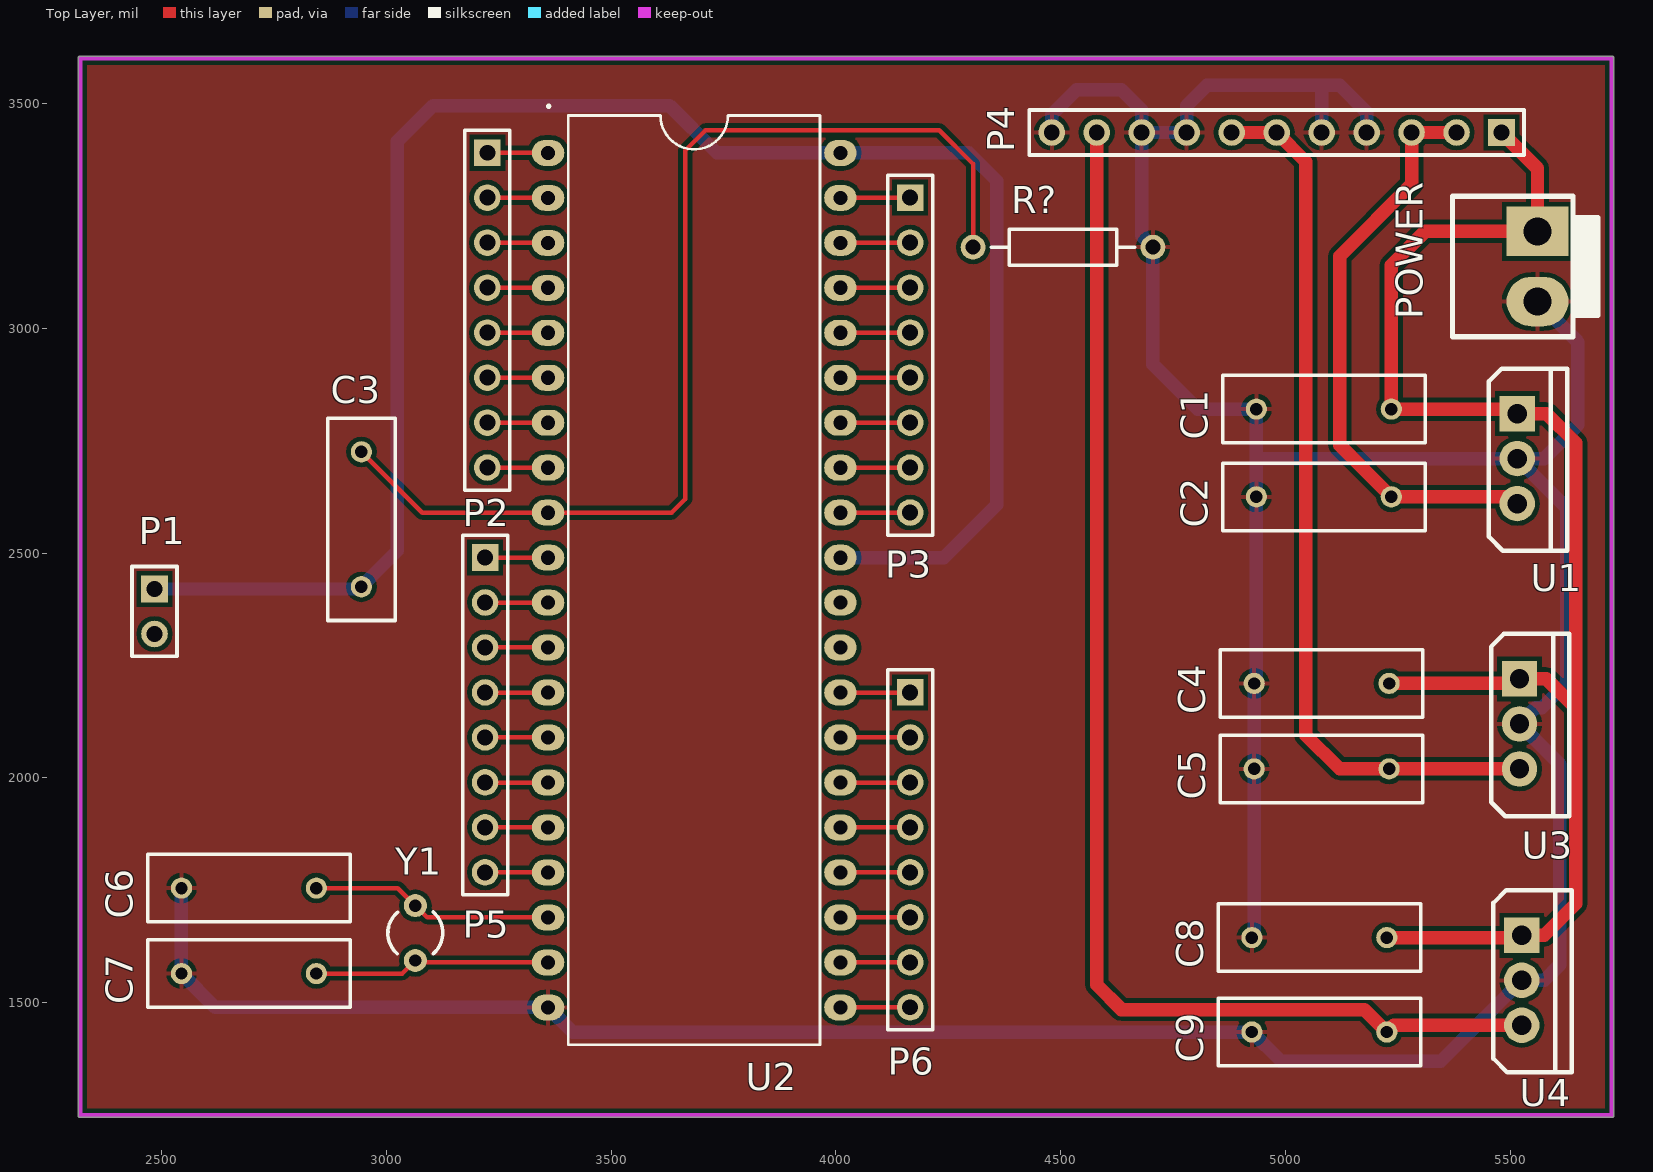
[diagram p0: Top Layer view]
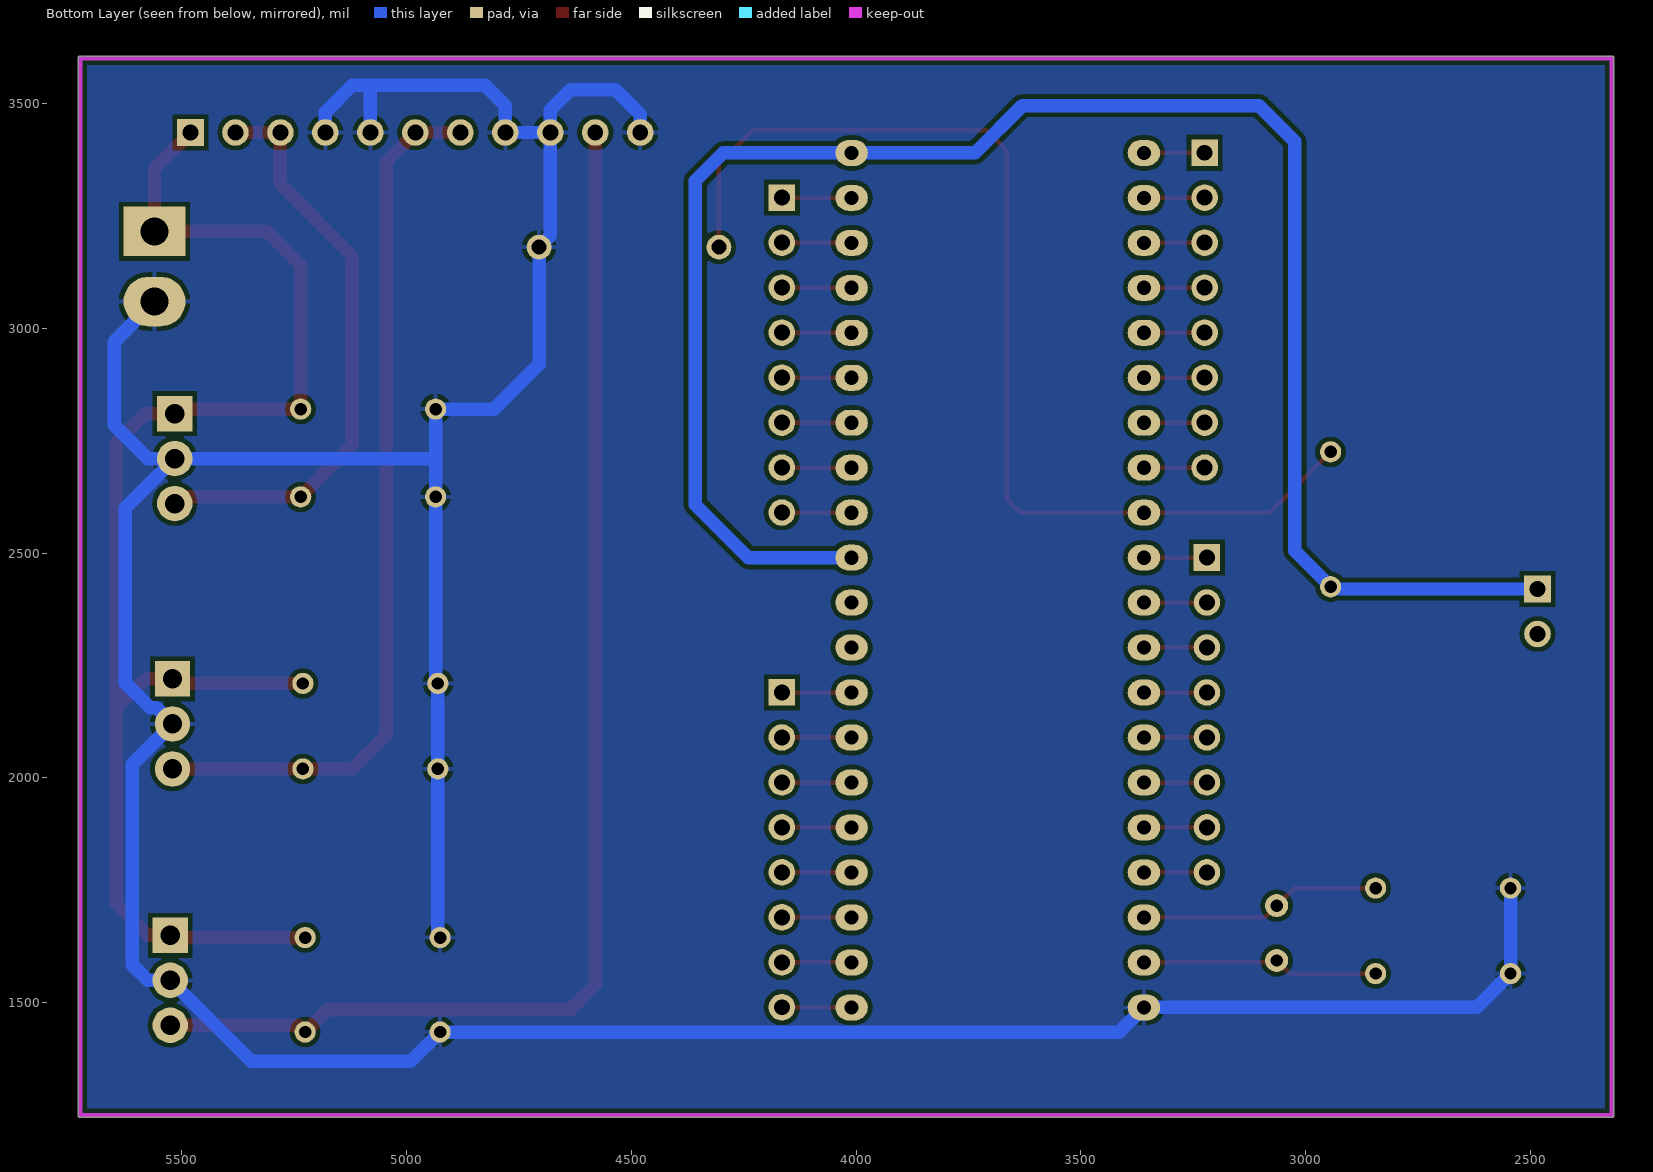
[diagram p1: Bottom Layer view, seen from below]
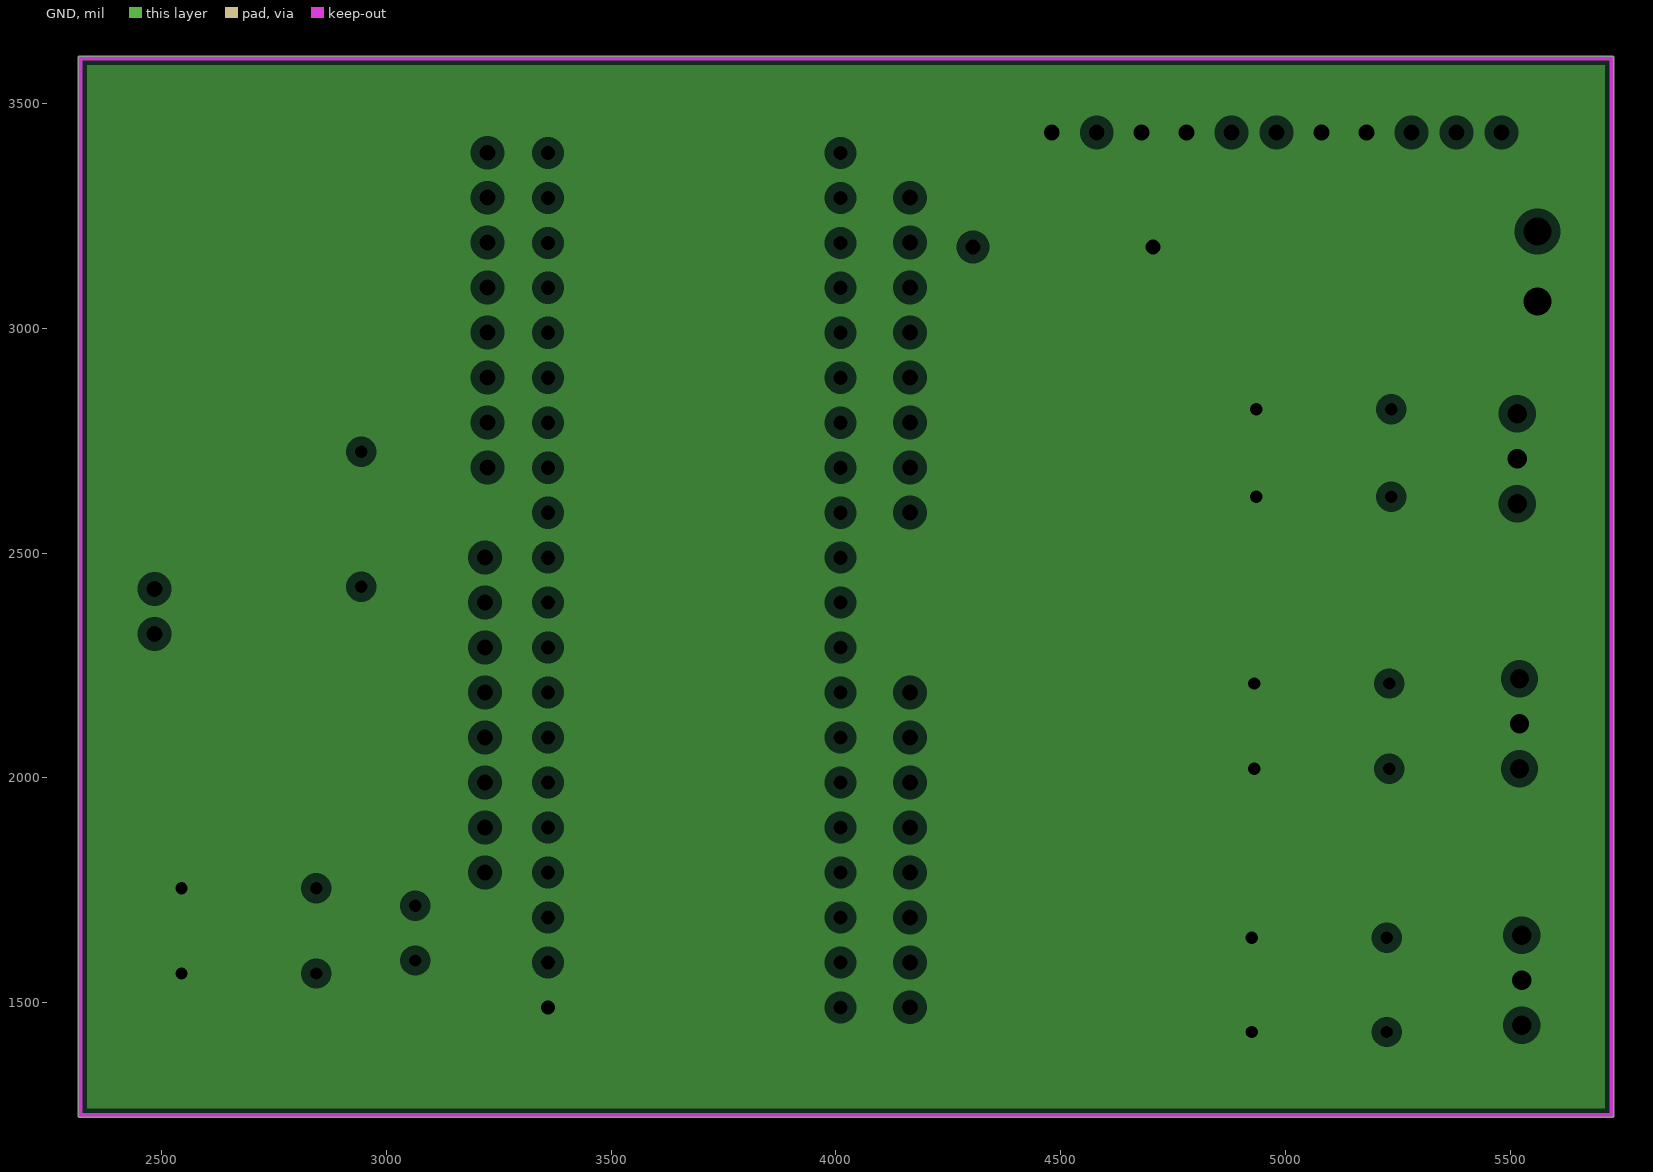
[diagram p2: GND, clearances drawn from the general rule]
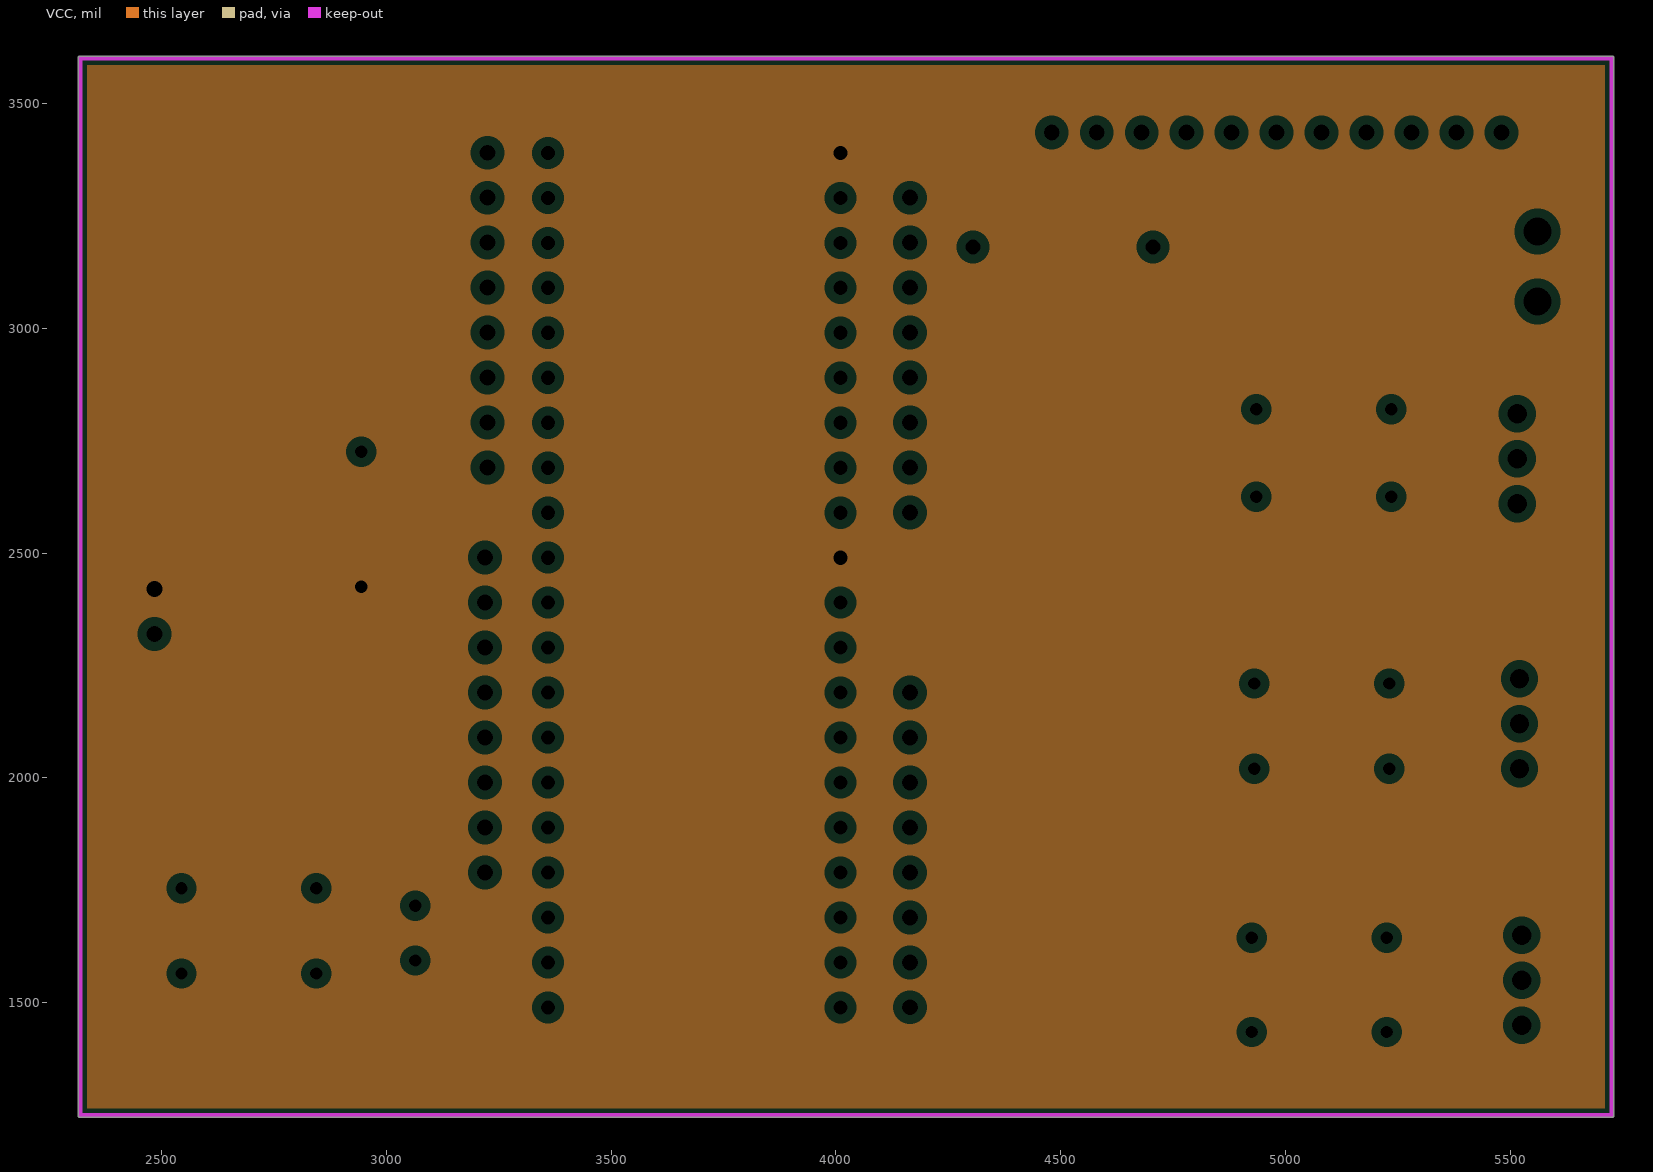
[diagram p3: VCC, clearances drawn from the general rule]
# Altium PCB MISC80518.PcbDoc
Units mil, origin at the board's own origin, x right, y up, seen from the top; angles counter-clockwise.
Board outline 3415.03 x 2360.03 mil, 4 copper layers (Top Layer, GND, VCC, Bottom Layer), stack 30.634 mil thick; 22 components, 41 nets, 118 pads, 0 vias.

## Layer stack, top to bottom
Top Solder: solder mask 0.4, Solder Resist, Dk 3.5
Top Layer: signal copper 1.4
Dielectric 1: core 10, FR-4, Dk 4.2
GND: plane copper 1.417, net GND
Dielectric 3: prepreg 5, Dk 4.2
VCC: plane copper 1.417, net VCC
Dielectric 2: core 10, Dk 4.2
Bottom Layer: signal copper 1.4
Bottom Solder: solder mask 0.4, Solder Resist, Dk 3.5

## Board outline
2314.99,1250 ccw(c2320,1250) 2320,1244.98 5725,1244.98 ccw(c5725,1250) 5730.02,1250 5730.02,3600 ccw(c5725,3600) 5725,3605.01 2320,3605.01 ccw(c2320,3600) 2314.99,3600

## Design rules (kind name [scope] priority, off if disabled: settings)
Clearance [All] p1: gap=10
MinimumSolderMaskSliver [All] p1: minsoldermaskwidth=0
PlaneClearance [All] p1: clearance=20
PlaneConnect [All] p1: planeconnectstyle=Relief reliefexpansion=20 reliefentries=4 reliefconductorwidth=10 reliefairgap=10
PolygonConnect [All] p1: connectstyle=Relief reliefconductorwidth=10 reliefentries=4 polygonreliefangle="90 Angle" airgapwidth=10
RoutingVias [All] p1: holewidth=28 width=50 viastyle="Through Hole" minholewidth=28 minwidth=50 maxholewidth=28 maxwidth=50
SilkToSilkClearance [All] p1: silktosilkclearance=0
SilkToSolderMaskClearance [IsPad] p1: minsilkscreentomaskgap=0 clearancetoexposedcopper=TRUE
SolderMaskExpansion [All] p1: expansion=4
Width [All] p1: maxlimit=50 minlimit=10 preferedwidth=10
25 further rules are at their usual default settings.

## Components (designator, comment, footprint, x,y, rotation, side; value= is the part's Value field where it differs from the comment)
C1 "0.33UF" RAD-0.3 5085,2820 r180 top
C2 "0.1UF" RAD-0.3 5085,2625 r180 top
C3 "10UF" RAD-0.3 2945,2575 r90 top
C4 "0.33UF" RAD-0.3 5080,2210 r180 top
C5 "0.1UF" RAD-0.3 5080,2020 r180 top
C6 "22pF" RAD-0.3 2695,1755 r180 top
C7 "22pF" RAD-0.3 2695,1565 r180 top
C8 "0.33UF" RAD-0.3 5075,1645 r180 top
C9 "0.1UF" RAD-0.3 5075,1435 r180 top
P1 "Header 2" HDR1X2 2485,2420 r270 top
P2 "Header 8" HDR1X8 3225,3390 r270 top
P3 "Header 8" HDR1X8 4165,3290 r270 top
P4 "Header 11" HDR1X11 5480,3435 r180 top
P5 "Header 8" HDR1X8 3220,2490 r270 top
P6 "Header 8" HDR1X8 4165,2190 r270 top
POWER "Terminal block" VH3.96-2A 5560,3215 r270 top
R? "10K" AXIAL-0.4 4505,3180 r180 top
U1 "LM7805" TO220A 5515,2710 r270 top
U2 "STC89C52RC" STC89C52RC 3685,2450 r270 top
U3 "LM7805" TO220A 5520,2120 r270 top
U4 "LM7806" TO220A 5525,1550 r270 top
Y1 "XTAL" R38 3065,1655 r180 top

## Footprints (in the part's own frame and the unit in brackets; to place one, negate y for a bottom-side part, rotate by r counter-clockwise, add the part's x,y. Pads: shape width x height; smd on the part's side, far side on the other; paste and mask are expansions set on the pad)
AXIAL-0.4 [mm] "Axial Device, Thru-Hole; 2 Leads; 0.4 in Pin Spacing"
  round 1.4 hole 0.85: 1(-5.08,0) 2(5.08,0)
  silkscreen extent -4.06,-1.02 4.06,1.02
HDR1X2 [mm] "Connector; Header; 2 Position"
  rect 1.5x1.5 hole 0.9: 1(0,0)
  round 1.5 hole 0.9: 2(2.54,0)
  silkscreen extent -1.27,-1.27 3.81,1.27
HDR1X8 [mm] "Connector; Header; 8 Position"
  rect 1.5x1.5 hole 0.9: 1(0,0)
  round 1.5 hole 0.9: 2(2.54,0) 3(5.08,0) 4(7.62,0) 5(10.16,0) 6(12.7,0) 7(15.24,0) 8(17.78,0)
  silkscreen extent -1.27,-1.27 19.05,1.27
HDR1X11 [mm] "Connector; Header; 11 Position"
  rect 1.5x1.5 hole 0.9: 1(0,0)
  round 1.5 hole 0.9: 2(2.54,0) 3(5.08,0) 4(7.62,0) 5(10.16,0) 6(12.7,0) 7(15.24,0) 8(17.78,0) 9(20.32,0) 10(22.86,0) 11(25.4,0)
  silkscreen extent -1.27,-1.27 26.67,1.27
R38 [mm] "Crystal, Thru-Hole; 2 Leads; Body 3.1 x 8.2 mm (Dia.xH)"
  round 1.3 hole 0.7: 1(0,1.55) 2(0,-1.55)
  silkscreen extent -1.55,-1.19 1.55,1.17
RAD-0.3 [mm] "Radial Cap, Thru-Hole; 2 Leads; 0.3 in Pin Spacing"
  round 1.2 hole 0.7: 1(-3.81,0) 2(3.81,0)
  silkscreen extent -5.71,-1.91 5.71,1.91
STC89C52RC [mm]
  oval 1.467x1.833 hole 0.8 paste+0 mask+0.051: 1(-23.868,-8.255) 2(-21.328,-8.255) 3(-18.788,-8.255) 4(-16.248,-8.255) 5(-13.708,-8.255) 6(-11.168,-8.255) 7(-8.628,-8.255) 8(-6.088,-8.255) 9(-3.548,-8.255) 10(-1.008,-8.255) 11(1.532,-8.255) 12(4.072,-8.255) 13(6.612,-8.255) 14(9.152,-8.255) 15(11.692,-8.255) 16(14.232,-8.255) 17(16.772,-8.255) 18(19.312,-8.255) 19(21.852,-8.255) 20(24.392,-8.255) 21(24.392,8.255) 22(21.852,8.255) 23(19.312,8.255) 24(16.772,8.255) 25(14.232,8.255) 26(11.692,8.255) 27(9.152,8.255) 28(6.612,8.255) 29(4.072,8.255) 30(1.532,8.255) 31(-1.008,8.255) 32(-3.548,8.255) 33(-6.088,8.255) 34(-8.628,8.255) 35(-11.168,8.255) 36(-13.708,8.255) 37(-16.248,8.255) 38(-18.788,8.255) 39(-21.328,8.255) 40(-23.868,8.255)
  silkscreen extent -26.58,-8.3 26.5,7.11
TO220A [mm] "220，3脚晶体管"
  rect 2x2 hole 1.1: 1(-2.54,0)
  round 2 hole 1.1: 2(0,0) 3(2.54,0)
  silkscreen extent -5.08,-1.6 5.21,2.82, body extent -5.08,-1.45 5.22,2.98, height 18.5
VH3.96-2A [mm]
  rect 2.8x3.5 hole 1.6: 1(0,0)
  oval 2.8x3.5 hole 1.6: 2(3.96,0)
  silkscreen extent -1.98,-4.8 5.94,3.4, body extent -1.98,-4.8 5.94,3.6, height 14.6

## Part data
C1 C2 C3 C4 C5 C6 C7 C8 C9: library part Cap, "Capacitor"
P1: "Header, 2-Pin"
P2 P3 P5 P6: "Header, 8-Pin"
P4: "Header, 11-Pin"
POWER: library part VH2
R?: library part Res2, "Resistor"
U4: library part LM7805
Y1: "Crystal Oscillator"

## Nets (pads, with @x,y where several pads share a name; then routed paths per layer and width w, separated by ;. In a path a pad name is that pad's centre, name@x,y a point inside that pad or via, vN(x,y) a via of type N, cw(c..) or ccw(c..) an arc to the next point about the centre after c; other vN are vias at no path point)
5V1: C2.1 P4.2 P4.3 U1.3 | length 1310.1
  Top Layer w30: P4.2 P4.3 5280,3320 5120,3160 5120,2740 C2.1 5500,2625 U1.3
5V2: C5.1 P4.6 P4.7 U3.3 | length 1973
  Top Layer w30: P4.7 P4.6 5045,3370 5045,2095 5120,2020 C5.1 U3.3
6V: C9.1 P4.10 U4.3 | length 2889.7
  Top Layer w30: P4.10 4580,1540 4635,1485 5175,1485 C9.1 5240,1450 U4.3
GND: C1.2 C2.2 C4.2 C5.2 C6.2 C7.2 C8.2 C9.2 P4.4 P4.5 P4.8 P4.9 P4.11 POWER.2 R?.1 U1.2 U2.20 U3.2 U4.2 | length 8804.8
  Bottom Layer w30: C6.2 C7.2 2620.33,1489.67 U2.20 3414.67,1435 C9.2 4990,1370 5345,1370 U4.2 5575,1550 5610,1585 5610,2030 U3.2 5555.63,2155.63 5569.73,2155.63 5625,2210.9 5625,2600 U1.2 ; P4.11 4480,3475 4535,3530 4635,3530 4680,3485 P4.9 ; C8.2 4930,1650 C5.2 C4.2 4935,2215 C2.2 4935,2715 ; P4.5 5080,3540 ; P4.4 5180,3480 5120,3540 5080,3540 ; POWER.2 5650,2969.09 5650,2785 5575,2710 U1.2 ; P4.9 4680,3205 R?.1 4705,2920 4805,2820 C1.2 4935,2715 ; P4.9 P4.8 4780,3495 4825,3540 5080,3540 ; 4935,2715 4940,2710 U1.2
NetC1_1: C1.1 C4.1 C8.1 P4.1 POWER.1 U1.1 U3.1 U4.1 | length 3292.4
  Top Layer w30: C8.1 5520,1645 U4.1 5575,1650 5645,1720 5645,2155 ; C4.1 5510,2210 U3.1 5580,2220 5645,2155 ; P4.1 5560,3355 POWER.1 5310,3215 5235,3140 C1.1 5505,2820 U1.1 5580,2810 5645,2745 5645,2155
NetC3_2: C3.2 R?.2 U2.9 | length 2438.3
  Top Layer w10: C3.2 3080.33,2589.67 U2.9 3634.67,2589.67 3665,2620 3665,3395 3710,3440 4230,3440 4305,3365 R?.2
NetC6_1: C6.1 U2.18 Y1.2 | length 542.1
  Top Layer w10: C6.1 3026.02,1755 Y1.2 3091.35,1689.67 U2.18
NetC7_1: C7.1 U2.19 Y1.1 | length 528.8
  Top Layer w10: C7.1 3036.02,1565 Y1.1 3069.31,1589.67 U2.19
NetP2_1: P2.1 U2.1 | length 135.1
  Top Layer w10: P2.1 3359.67,3390 U2.1
NetP2_2: P2.2 U2.2 | length 135.1
  Top Layer w10: P2.2 3225.33,3289.67 U2.2
NetP2_3: P2.3 U2.3 | length 135.1
  Top Layer w10: P2.3 3359.67,3190 U2.3
NetP2_4: P2.4 U2.4 | length 135.1
  Top Layer w10: P2.4 3225.33,3089.67 U2.4
NetP2_5: P2.5 U2.5 | length 135.1
  Top Layer w10: P2.5 3359.67,2990 U2.5
NetP2_6: P2.6 U2.6 | length 135.1
  Top Layer w10: P2.6 3359.67,2890 U2.6
NetP2_7: P2.7 U2.7 | length 135.1
  Top Layer w10: P2.7 3225.33,2789.67 U2.7
NetP2_8: P2.8 U2.8 | length 135.1
  Top Layer w10: P2.8 3359.67,2690 U2.8
NetP3_1: P3.1 U2.39 | length 155.1
  Top Layer w10: U2.39 4164.67,3289.67 P3.1
NetP3_2: P3.2 U2.38 | length 155.1
  Top Layer w10: U2.38 4010.33,3190 P3.2
NetP3_3: P3.3 U2.37 | length 155.1
  Top Layer w10: U2.37 4164.67,3089.67 P3.3
NetP3_4: P3.4 U2.36 | length 155.1
  Top Layer w10: U2.36 4164.67,2989.67 P3.4
NetP3_5: P3.5 U2.35 | length 155.1
  Top Layer w10: U2.35 4010.33,2890 P3.5
NetP3_6: P3.6 U2.34 | length 155.1
  Top Layer w10: U2.34 4164.67,2789.67 P3.6
NetP3_7: P3.7 U2.33 | length 155.1
  Top Layer w10: U2.33 4010.33,2690 P3.7
NetP3_8: P3.8 U2.32 | length 155.1
  Top Layer w10: U2.32 4164.67,2589.67 P3.8
NetP5_1: P5.1 U2.10 | length 140.1
  Top Layer w10: P5.1 3359.67,2490 U2.10
NetP5_2: P5.2 U2.11 | length 140.1
  Top Layer w10: P5.2 3220.33,2389.67 U2.11
NetP5_3: P5.3 U2.12 | length 140.1
  Top Layer w10: P5.3 3359.67,2290 U2.12
NetP5_4: P5.4 U2.13 | length 140.1
  Top Layer w10: P5.4 3220.33,2189.67 U2.13
NetP5_5: P5.5 U2.14 | length 140.1
  Top Layer w10: P5.5 3359.67,2090 U2.14
NetP5_6: P5.6 U2.15 | length 140.1
  Top Layer w10: P5.6 3220.33,1989.67 U2.15
NetP5_7: P5.7 U2.16 | length 140.1
  Top Layer w10: P5.7 3359.67,1890 U2.16
NetP5_8: P5.8 U2.17 | length 140.1
  Top Layer w10: P5.8 3220.33,1789.67 U2.17
NetP6_1: P6.1 U2.28 | length 155.1
  Top Layer w10: U2.28 4164.67,2189.67 P6.1
NetP6_2: P6.2 U2.27 | length 155.1
  Top Layer w10: U2.27 4010.33,2090 P6.2
NetP6_3: P6.3 U2.26 | length 155.1
  Top Layer w10: U2.26 4164.67,1989.67 P6.3
NetP6_4: P6.4 U2.25 | length 155.1
  Top Layer w10: U2.25 4010.33,1890 P6.4
NetP6_5: P6.5 U2.24 | length 155.1
  Top Layer w10: U2.24 4164.67,1789.67 P6.5
NetP6_6: P6.6 U2.23 | length 155.1
  Top Layer w10: U2.23 4164.67,1689.67 P6.6
NetP6_7: P6.7 U2.22 | length 155.1
  Top Layer w10: U2.22 4010.33,1590 P6.7
NetP6_8: P6.8 U2.21 | length 155.1
  Top Layer w10: U2.21 4164.67,1489.67 P6.8
VCC: C3.1 P1.1 U2.31 U2.40 | length 4036.6
  Bottom Layer w30: P1.1 2940,2420 C3.1 3025,2505 3025,3415 3105,3495 3630,3495 3735.33,3389.67 U2.40 4295.33,3389.67 4357.56,3327.44 4357.56,2607.56 4239.67,2489.67 U2.31
pads on no net: P1.2 U2.29 U2.30

## Polygon pours and split planes (outlines as drawn)
GND on Top Layer "D" (solid, remove dead copper, pour order 0): 1765,3900 6190,3900 6220,3930 6035,3745 6035,1175 2125,1175 2020,1070
GND on Bottom Layer "D" (solid, remove dead copper, pour order 2): 1850,3895 1960,4005 5825,4005 5825,1195 6070,950 6035,985 1755,985
GND on GND (split plane): 5709.92,1265.08 2335.08,1265.08 2335.08,3584.92 5709.92,3584.92
VCC on VCC (split plane): 5709.92,1265.08 2335.08,1265.08 2335.08,3584.92 5709.92,3584.92

## Keep-outs
Keep-Out Layer:
  lines w10: 2400,3600 5725,3600 5725,1250 2320,1250 2320,2745 2320,3600 2420,3600